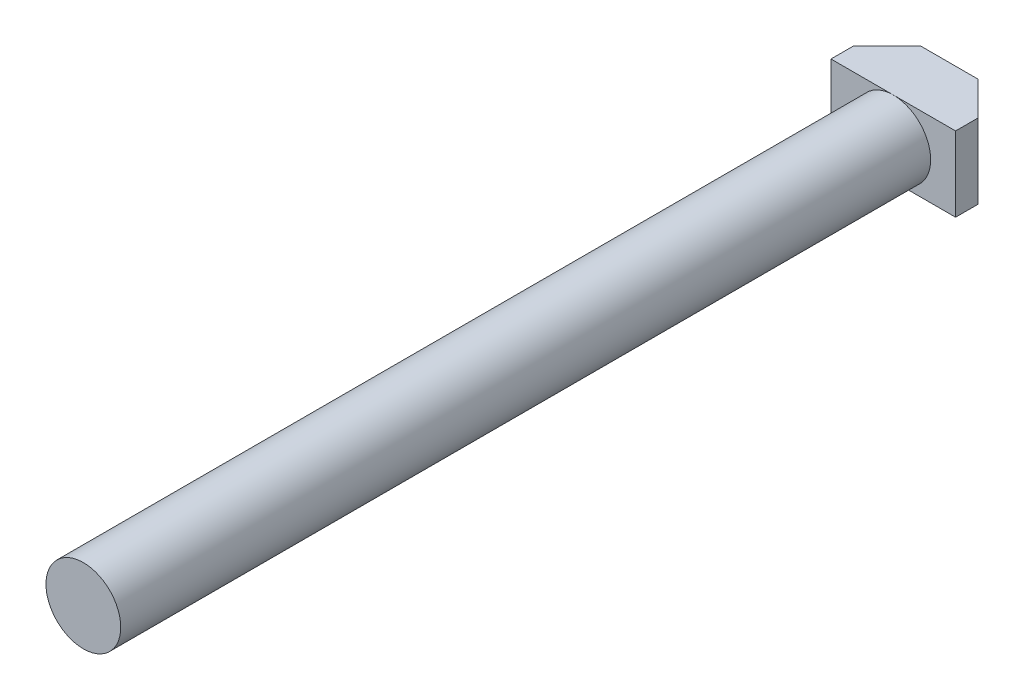
from build123d import *

# Parameters (mm, degrees)
BOSS_EXTRUDE1_DEPTH = 6
SKETCH2_R           = 3
BOSS_EXTRUDE2_DEPTH = 65


with BuildPart() as part:
    # Sketch1 → Boss-Extrude1 (new body)
    with BuildSketch(Plane(origin=(0, 0, 0), x_dir=(1, 0, 0), z_dir=(0, 1, 0))):
        Polygon((-6.879699248, 12.868308957), (3.120300752, 12.868308957), (3.120300752, 14.668308957), (0.420300752, 17.368308957), (-4.179699248, 17.368308957), (-6.879699248, 14.668308957), align=None)
    extrude(amount=BOSS_EXTRUDE1_DEPTH)

    # Sketch2 → Boss-Extrude2 (add)
    with BuildSketch(Plane.XY.offset(-12.868308957)):
        with Locations(Location((-1.879699248, 3, 0), (0, 0, 270))):
            Circle(SKETCH2_R)
    extrude(amount=BOSS_EXTRUDE2_DEPTH)


solid = part.part
